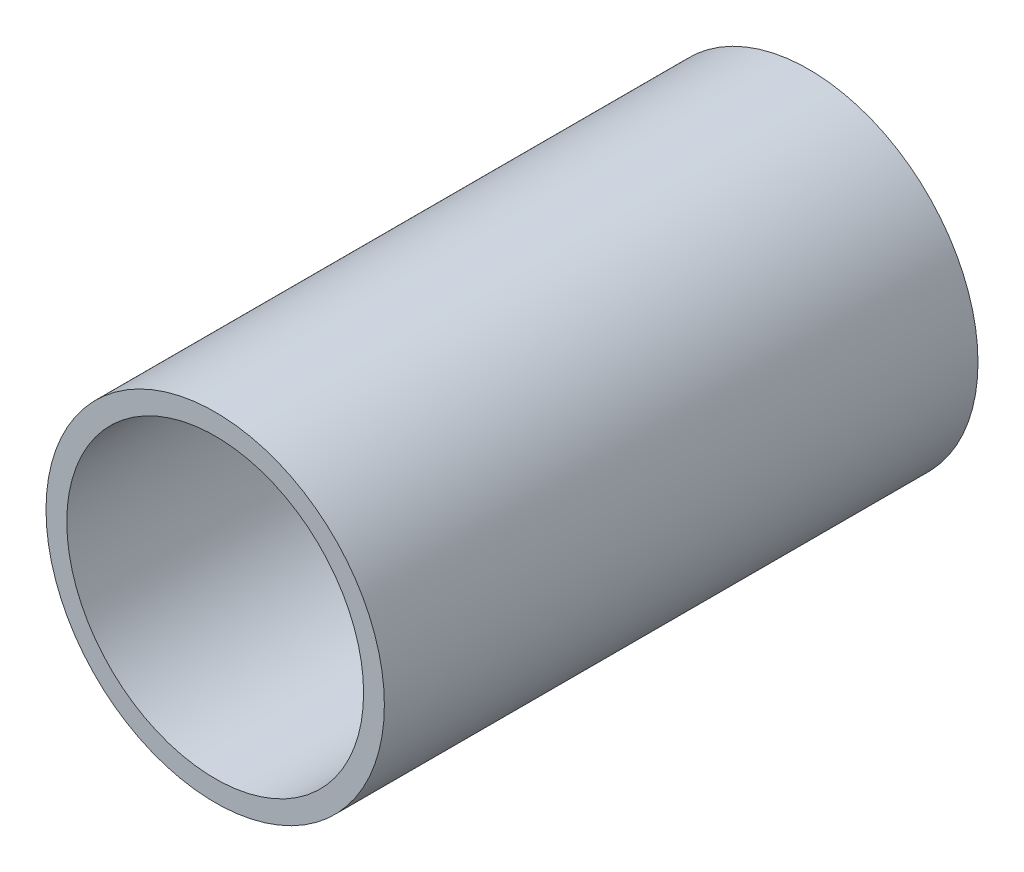
from build123d import *

# Parameters (mm, degrees)
SKETCH1_R           = 57
SKETCH1_R_2         = 50
BOSS_EXTRUDE1_DEPTH = 200


with BuildPart() as part:
    # Sketch1 → Boss-Extrude1 (new body)
    with BuildSketch(Plane.XY):
        Circle(SKETCH1_R)
        Circle(SKETCH1_R_2, mode=Mode.SUBTRACT)
    extrude(amount=BOSS_EXTRUDE1_DEPTH)


solid = part.part
